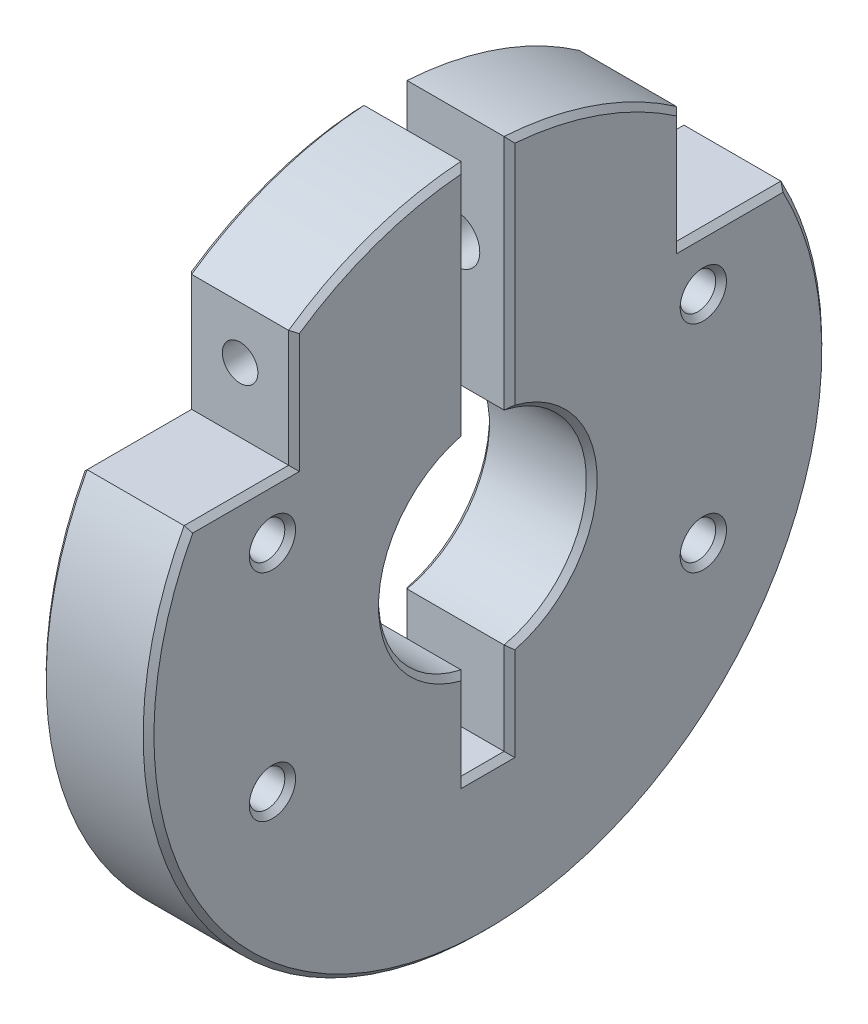
SolidWorks part; units mm, degrees
material "S45C"
ref_plane "Front Plane" through (0, 0, 0) normal (0, 0, 1) x (1, 0, 0)
ref_plane "Top Plane" through (0, 0, 0) normal (0, 1, 0) x (1, 0, 0)
ref_plane "Right Plane" through (0, 0, 0) normal (1, 0, 0) x (0, 0, -1)
sketch "Sketch1" plane through (0, 0, 0) normal (1, 0, 0) x (0, 0, -1)
  line L0 (0, -24.959) -> (0, 50.3964) construction
  line L1 (2, -9.4405) -> (2, -18)
  line L2 (-2, 31.4364) -> (-2, 9.4405)
  line L3 (-2, -18) -> (2, -18)
  line L4 (2, 31.4364) -> (2, 9.4405)
  line L5 (-2, -9.4405) -> (-2, -18)
  line L6 (-18, 25.8505) -> (-18, 15)
  line L7 (-18, 15) -> (-27.6993, 15)
  line L8 (18, 25.8505) -> (18, 15)
  line L9 (18, 15) -> (27.6993, 15)
  arc A0 (-2, 31.4364) -> (-18, 25.8505) centre (0, 0) ccw
  arc A1 (-2, 9.4405) -> (-2, -9.4405) centre (0, 0) ccw
  arc A2 (2, -9.4405) -> (2, 9.4405) centre (0, 0) ccw
  arc A3 (-27.6993, 15) -> (27.6993, 15) centre (0, 0) ccw
  arc A4 (18, 25.8505) -> (2, 31.4364) centre (0, 0) ccw
  dimension "D1" = 63
  dimension "D2" = 19.3
  dimension "D3" = 18
  dimension "D4" = 4
  dimension "D5" = 18
  dimension "D6" = 15
extrude "Boss-Extrude1" add sketch "Sketch1" along normal mid plane 10
hole_wizard "Hole size by socket head cap screw type1" positions "Sketch3" profile "Sketch2" counterbore size "M4" standard "Gb"
sketch "Sketch3" plane through (0, 0, -18) normal (0, 0, -1) x (-1, 0, 0)
  line L2 (0, 0) -> (0, 21) construction
  point P0 (0, 21)
  dimension "D1" = 21
sketch "Sketch2" plane through (0, 21, -18) normal (1, 0, 0) x (0, 1, 0)
  line L0 (0, 0) -> (0, 16)
  line L1 (0, 16) -> (2.25, 16)
  line L3 (2.25, 16) -> (2.25, 4.6)
  line L4 (2.25, 4.6) -> (4, 4.6)
  line L5 (4, 4.6) -> (4, 0)
  line L7 (4, 0) -> (0, 0)
  line L11 (0, -6.35) -> (0, 107.95) construction
  dimension "通孔孔直径" = 4.5
  dimension "通孔孔深度" = 16
  dimension "柱形沉头孔直径" = 8
  dimension "柱形沉头孔深度" = 4.6
hole_wizard "M4 Tapped Hole1" positions "Sketch5" profile "Sketch4" tap size "M4" standard "Gb" end condition through all
sketch "Sketch5" plane through (0, 0, 2) normal (0, 0, -1) x (-1, 0, 0)
  point P0 (0, 21)
sketch "Sketch4" plane through (0, 21, 2) normal (1, 0, 0) x (0, 1, 0)
  line L0 (0, 0) -> (0, 29.5)
  line L1 (0, 29.5) -> (1.65, 29.5)
  line L2 (1.65, 29.5) -> (1.65, 0)
  line L5 (1.65, 0) -> (0, 0)
  line L11 (0, -6.35) -> (0, 107.95) construction
  dimension "通孔螺纹孔钻头直径" = 3.3
  dimension "通孔螺纹孔钻头深度" = 29.5
cosmetic thread "Cosmetic Thread1" parameters "D2"=4
hole_wizard "M4 Tapped Hole2" positions "Sketch7" profile "Sketch6" tap size "M4" standard "Gb" end condition through all
sketch "Sketch7" plane through (5, 0, 0) normal (1, 0, 0) x (0, 0, -1)
  line L0 (0, 23.281) -> (0, -29.9882) construction
  line L4 (-25.5748, 0) -> (26.3703, 0) construction
  point P0 (20, 10)
  point P2 (20, -10)
  point P4 (-20, -10)
  point P6 (-20, 10)
  dimension "D1" = 20
  dimension "D2" = 40
sketch "Sketch6" plane through (5, 10, -20) normal (0, 1, 0) x (0, 0, -1)
  line L0 (0, 0) -> (0, 10)
  line L1 (0, 10) -> (1.65, 10)
  line L2 (1.65, 10) -> (1.65, 0)
  line L5 (1.65, 0) -> (0, 0)
  line L11 (0, -6.35) -> (0, 107.95) construction
  dimension "通孔螺纹孔钻头直径" = 3.3
  dimension "通孔螺纹孔钻头深度" = 10
cosmetic thread "Cosmetic Thread2" parameters "D2"=4
cosmetic thread "Cosmetic Thread3" parameters "D2"=4
cosmetic thread "Cosmetic Thread4" parameters "D2"=4
cosmetic thread "Cosmetic Thread5" parameters "D2"=4
chamfer "Chamfer1" distance 0.5 angle 45 40 edges at (-5, 20.4385, -2) (-5, 0, -9.65) (-5, -13.7202, -2) (-5, -18, 0) (-5, -13.7202, 2) (-5, 0, 9.65) (-5, 20.4385, 2) (-5, 29.7397, 10.3827) (-5, 20.4253, 18) (-5, 15, 22.8496) (-5, -31.5, 0) (-5, 15, -22.8496) (-5, 20.4253, -18) (-5, 29.7397, -10.3827) (-5, 10, 18.35) (-5, -10, 18.35) (-5, -10, -21.65) (-5, 10, -21.65) (5, 20.4253, -18) (5, 15, -22.8496) (5, -31.5, 0) (5, 15, 22.8496) (5, 20.4253, 18) (5, 29.7397, 10.3827) (5, 20.4385, 2) (5, 0, 9.65) (5, -13.7202, 2) (5, -18, 0) (5, -13.7202, -2) (5, 0, -9.65) (5, 20.4385, -2) (5, 29.7397, -10.3827) (5, 10, 18.35) (5, -10, 18.35) (5, -10, -21.65) (5, 10, -21.65) (0, 15, -27.6993) (0, 15, 27.6993) (0, 25.8505, 18) (0, 25.8505, -18)
